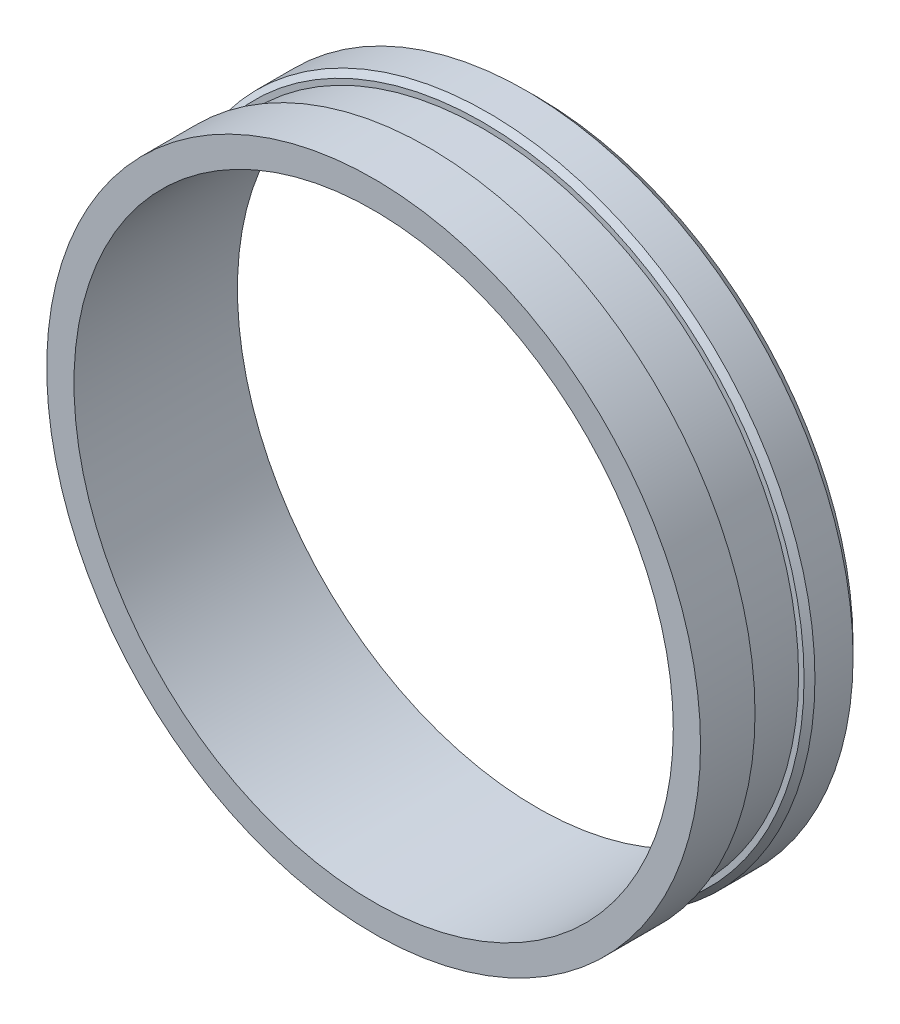
SolidWorks part; units mm, degrees
ref_plane "Front Plane" through (0, 0, 0) normal (0, 0, 1) x (1, 0, 0)
ref_plane "Top Plane" through (0, 0, 0) normal (0, 1, 0) x (1, 0, 0)
ref_plane "Right Plane" through (0, 0, 0) normal (1, 0, 0) x (0, 0, -1)
sketch "Sketch1" plane through (0, 0, 0) normal (0, 0, 1) x (1, 0, 0)
  circle A0 centre (0, 0) radius 60
  circle A1 centre (0, 0) radius 55
  dimension "D1" = 120
  dimension "D2" = 110
extrude "Boss-Extrude1" add sketch "Sketch1" along normal blind 20
sketch "Sketch2" plane through (0, 0, 20) normal (0, 0, 1) x (1, 0, 0)
  circle A0 centre (0, 0) radius 58
  circle A1 centre (0, 0) radius 60
  dimension "D1" = 116
extrude "Cut-Extrude1" cut sketch "Sketch2" against normal blind 10
sketch "Sketch3" plane through (0, 0, 20) normal (0, 0, 1) x (1, 0, 0)
  circle A0 centre (0, 0) radius 60
  circle A1 centre (0, 0) radius 55
extrude "Boss-Extrude2" add sketch "Sketch3" along normal blind 10
chamfer "Chamfer1" distance 2 1 edges at (60, 0, 0)
chamfer "Chamfer2" distance 1 1 edges at (60, 0, 10)
